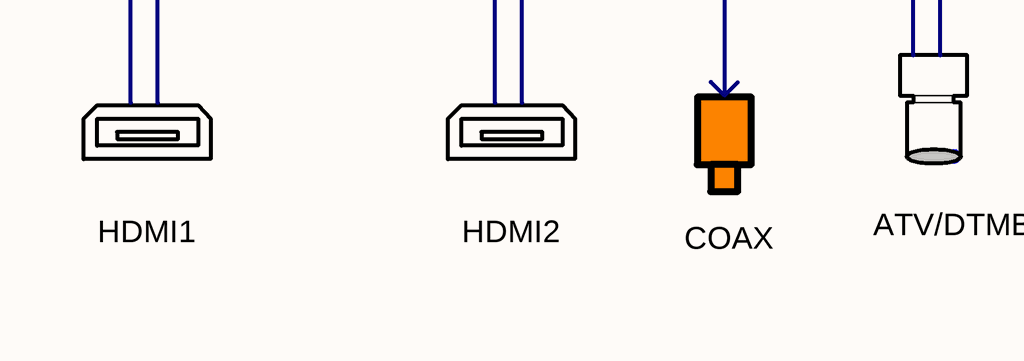
[diagram p0: MISC84395-2.schdoc, bottom right]
# Altium project MISC84395-37.PrjPCB (part 3 of 13)

## Sheet MISC84395-2.schdoc (continued)

### Notes on the sheet
- 3V3_M
- SYSTEM FUNCTION BLOCK DIAGRAM
- M_I2C
- AA7
- W6
- SI2159
- Panel
- Addr
- 348
- DCDC-SCL
- E4
- E5
- DCDC-SDA
- DCDC
- Main Board Power Tree
- KEYPAD
- IR
- LED
- LVDS&MLVDS
- DDR3
- PSU
- AMP_12
- 1800mA
- AD52050B
- 512MB*1
- 12V
- 5V_STB
- 5V_M
- 1200mA
- DC-DC
- UD2
- Approx. 2300mA
- 1900mA
- 460mA
- LDO
- UL1
- EMMC
- SY8113IADC
- PW_EN
- 80mA
- eMMC
- SOC
- 280mA
- 648
- Tuner
- 200mA
- 102/101
- flash
- 190mA
- 3V3_STB
- 230mA
- 40mA
- 1V8_M
- MS346T
- EMMC 1V8
- WIFI&BT
- SDIO
- 215mA
- SY8088IAAC
- 1V5_M_DDR
- 610mA
- WIFI
- 1*DDR
- 500mA
- USB2.0
- R
- AMP
- L
- 1000mA
- VCC-PANEL
- LVDS
- PENAL_EN
- 160mA
- 1.05V
- VDDC_CPU
- 1500mA
- RJ45
- USB 2.0
- CVBS & Audio IN
- HDMI1
- HDMI2
- COAX
- ATV/DTMB
- 250mA
- MSH6110A
- 1.1V
- 2400mA